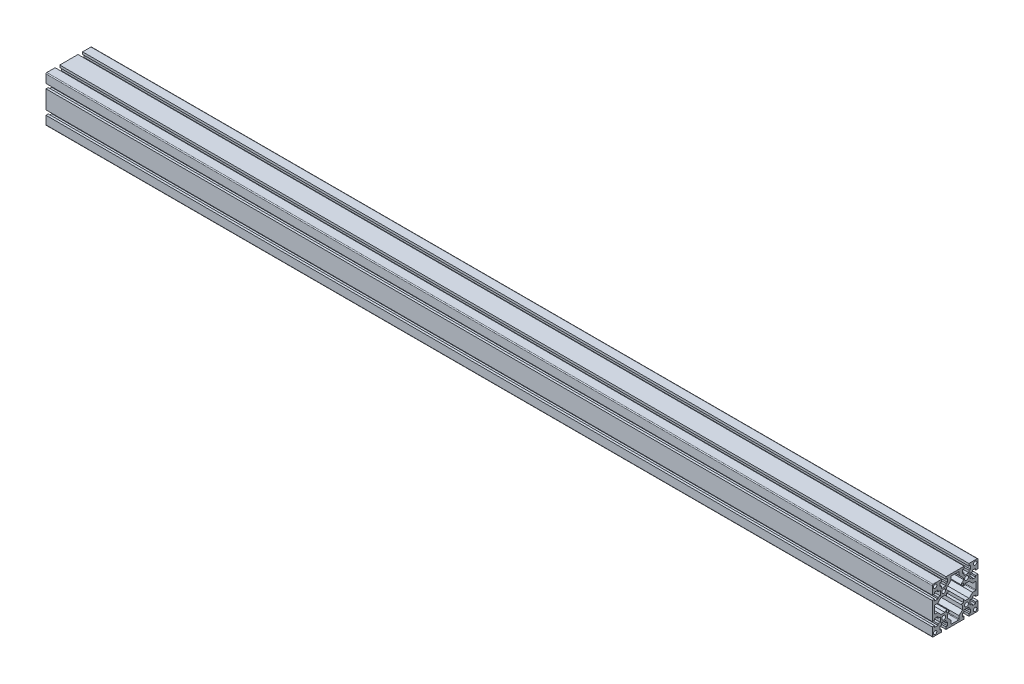
from build123d import *

# Parameters (mm, degrees)
SKETCH1_R                                 = 3.4
SKETCH1_R_2                               = 3
ALUMINIUM_PROFILE_80_X_80G_X_R1_5_1_DEPTH = 1550
SKETCH10_R                                = 3
CUT_EXTRUDE1_DEPTH                        = 1552.031914565


with BuildPart() as part:
    # Sketch1 → Aluminium profile 80 X 80G X R1.5(1) (new body)
    with BuildSketch(Plane.YZ.offset(-530.344827586)):
        with BuildLine():
            Line((-24.05, 40), (-24.05, 36))
            Line((-24.05, 36), (-26.75, 36))
            Line((-26.75, 36), (-26.75, 30))
            Line((-26.75, 30), (-24.05, 30))
            Line((-24.05, 30), (-24.05, 26))
            Line((-24.05, 26), (-15.95, 26))
            Line((-15.95, 26), (-15.95, 30))
            Line((-15.95, 30), (-13.25, 30))
            Line((-13.25, 30), (-13.25, 36))
            Line((-13.25, 36), (-15.95, 36))
            Line((-15.95, 36), (-15.95, 40))
            Line((-15.95, 40), (15.95, 40))
            Line((15.95, 40), (15.95, 36))
            Line((15.95, 36), (13.25, 36))
            Line((13.25, 36), (13.25, 30))
            Line((13.25, 30), (15.95, 30))
            Line((15.95, 30), (15.95, 26))
            Line((15.95, 26), (24.05, 26))
            Line((24.05, 26), (24.05, 30))
            Line((24.05, 30), (26.75, 30))
            Line((26.75, 30), (26.75, 36))
            Line((26.75, 36), (24.05, 36))
            Line((24.05, 36), (24.05, 40))
            Line((24.05, 40), (38.5, 40))
            ThreePointArc((38.5, 40), (39.560660172, 39.560660172), (40, 38.5))
            Line((40, 38.5), (40, 24.05))
            Line((40, 24.05), (36, 24.05))
            Line((36, 24.05), (36, 26.75))
            Line((36, 26.75), (30, 26.75))
            Line((30, 26.75), (30, 24.05))
            Line((30, 24.05), (26, 24.05))
            Line((26, 24.05), (26, 15.95))
            Line((26, 15.95), (30, 15.95))
            Line((30, 15.95), (30, 13.25))
            Line((30, 13.25), (36, 13.25))
            Line((36, 13.25), (36, 15.95))
            Line((36, 15.95), (40, 15.95))
            Line((40, 15.95), (40, -15.95))
            Line((40, -15.95), (36, -15.95))
            Line((36, -15.95), (36, -13.25))
            Line((36, -13.25), (30, -13.25))
            Line((30, -13.25), (30, -15.95))
            Line((30, -15.95), (26, -15.95))
            Line((26, -15.95), (26, -24.05))
            Line((26, -24.05), (30, -24.05))
            Line((30, -24.05), (30, -26.75))
            Line((30, -26.75), (36, -26.75))
            Line((36, -26.75), (36, -24.05))
            Line((36, -24.05), (40, -24.05))
            Line((40, -24.05), (40, -38.5))
            ThreePointArc((40, -38.5), (39.560660172, -39.560660172), (38.5, -40))
            Line((38.5, -40), (24.05, -40))
            Line((24.05, -40), (24.05, -36))
            Line((24.05, -36), (26.75, -36))
            Line((26.75, -36), (26.75, -30))
            Line((26.75, -30), (24.05, -30))
            Line((24.05, -30), (24.05, -26))
            Line((24.05, -26), (15.95, -26))
            Line((15.95, -26), (15.95, -30))
            Line((15.95, -30), (13.25, -30))
            Line((13.25, -30), (13.25, -36))
            Line((13.25, -36), (15.95, -36))
            Line((15.95, -36), (15.95, -40))
            Line((15.95, -40), (-15.95, -40))
            Line((-15.95, -40), (-15.95, -36))
            Line((-15.95, -36), (-13.25, -36))
            Line((-13.25, -36), (-13.25, -30))
            Line((-13.25, -30), (-15.95, -30))
            Line((-15.95, -30), (-15.95, -26))
            Line((-15.95, -26), (-24.05, -26))
            Line((-24.05, -26), (-24.05, -30))
            Line((-24.05, -30), (-26.75, -30))
            Line((-26.75, -30), (-26.75, -36))
            Line((-26.75, -36), (-24.05, -36))
            Line((-24.05, -36), (-24.05, -40))
            Line((-24.05, -40), (-38.5, -40))
            ThreePointArc((-38.5, -40), (-39.560660172, -39.560660172), (-40, -38.5))
            Line((-40, -38.5), (-40, -24.05))
            Line((-40, -24.05), (-36, -24.05))
            Line((-36, -24.05), (-36, -26.75))
            Line((-36, -26.75), (-30, -26.75))
            Line((-30, -26.75), (-30, -24.05))
            Line((-30, -24.05), (-26, -24.05))
            Line((-26, -24.05), (-26, -15.95))
            Line((-26, -15.95), (-30, -15.95))
            Line((-30, -15.95), (-30, -13.25))
            Line((-30, -13.25), (-36, -13.25))
            Line((-36, -13.25), (-36, -15.95))
            Line((-36, -15.95), (-40, -15.95))
            Line((-40, -15.95), (-40, 15.95))
            Line((-40, 15.95), (-36, 15.95))
            Line((-36, 15.95), (-36, 13.25))
            Line((-36, 13.25), (-30, 13.25))
            Line((-30, 13.25), (-30, 15.95))
            Line((-30, 15.95), (-26, 15.95))
            Line((-26, 15.95), (-26, 24.05))
            Line((-26, 24.05), (-30, 24.05))
            Line((-30, 24.05), (-30, 26.75))
            Line((-30, 26.75), (-36, 26.75))
            Line((-36, 26.75), (-36, 24.05))
            Line((-36, 24.05), (-40, 24.05))
            Line((-40, 24.05), (-40, 38.5))
            ThreePointArc((-40, 38.5), (-39.560660172, 39.560660172), (-38.5, 40))
            Line((-38.5, 40), (-24.05, 40))
        make_face()
        with Locations((-20, 20)):
            Circle(SKETCH1_R, mode=Mode.SUBTRACT)
        with Locations((20, 20)):
            Circle(SKETCH1_R, mode=Mode.SUBTRACT)
        with Locations((20, -20)):
            Circle(SKETCH1_R, mode=Mode.SUBTRACT)
        with Locations((-20, -20)):
            Circle(SKETCH1_R, mode=Mode.SUBTRACT)
        with Locations((-35, 35)):
            Circle(SKETCH1_R_2, mode=Mode.SUBTRACT)
        with Locations((35, 35)):
            Circle(SKETCH1_R_2, mode=Mode.SUBTRACT)
        with Locations((35, -35)):
            Circle(SKETCH1_R_2, mode=Mode.SUBTRACT)
        with BuildLine():
            Line((-13, 18), (-10, 15))
            Line((-10, 15), (-15, 15))
            Line((-15, 15), (-15, 10))
            Line((-15, 10), (-18, 13))
            Line((-18, 13), (-24.5, 13))
            Line((-24.5, 13), (-30.5, 7))
            Line((-30.5, 7), (-35.5, 7))
            ThreePointArc((-35.5, 7), (-36.207106781, 6.707106781), (-36.5, 6))
            Line((-36.5, 6), (-36.5, -6))
            ThreePointArc((-36.5, -6), (-36.207106781, -6.707106781), (-35.5, -7))
            Line((-35.5, -7), (-30.5, -7))
            Line((-30.5, -7), (-24.5, -13))
            Line((-24.5, -13), (-18, -13))
            Line((-18, -13), (-15, -10))
            Line((-15, -10), (-15, -15))
            Line((-15, -15), (-10, -15))
            Line((-10, -15), (-13, -18))
            Line((-13, -18), (-13, -24.5))
            Line((-13, -24.5), (-7, -30.5))
            Line((-7, -30.5), (-7, -35.5))
            ThreePointArc((-7, -35.5), (-6.707106781, -36.207106781), (-6, -36.5))
            Line((-6, -36.5), (6, -36.5))
            ThreePointArc((6, -36.5), (6.707106781, -36.207106781), (7, -35.5))
            Line((7, -35.5), (7, -30.5))
            Line((7, -30.5), (13, -24.5))
            Line((13, -24.5), (13, -18))
            Line((13, -18), (10, -15))
            Line((10, -15), (15, -15))
            Line((15, -15), (15, -10))
            Line((15, -10), (20, -15))
            Line((20, -15), (22.5, -15))
            Line((22.5, -15), (30.5, -7))
            Line((30.5, -7), (35.5, -7))
            ThreePointArc((35.5, -7), (36.207106781, -6.707106781), (36.5, -6))
            Line((36.5, -6), (36.5, 6))
            ThreePointArc((36.5, 6), (36.207106781, 6.707106781), (35.5, 7))
            Line((35.5, 7), (30.5, 7))
            Line((30.5, 7), (22.5, 15))
            Line((22.5, 15), (20, 15))
            Line((20, 15), (15, 10))
            Line((15, 10), (15, 15))
            Line((15, 15), (10, 15))
            Line((10, 15), (13, 18))
            Line((13, 18), (13, 24.5))
            Line((13, 24.5), (7, 30.5))
            Line((7, 30.5), (7, 35.5))
            ThreePointArc((7, 35.5), (6.707106781, 36.207106781), (6, 36.5))
            Line((6, 36.5), (-6, 36.5))
            ThreePointArc((-6, 36.5), (-6.707106781, 36.207106781), (-7, 35.5))
            Line((-7, 35.5), (-7, 30.5))
            Line((-7, 30.5), (-13, 24.5))
            Line((-13, 24.5), (-13, 18))
        make_face(mode=Mode.SUBTRACT)
    extrude(amount=ALUMINIUM_PROFILE_80_X_80G_X_R1_5_1_DEPTH)

    # Sketch10 → Cut-Extrude1 (cut, through all)
    with BuildSketch(Plane(origin=(1019.655172414, 0, 0), x_dir=(0, 0, -1), z_dir=(1, 0, 0))):
        with Locations((35, -35)):
            Circle(SKETCH10_R)
    extrude(amount=-CUT_EXTRUDE1_DEPTH, mode=Mode.SUBTRACT)


solid = part.part
